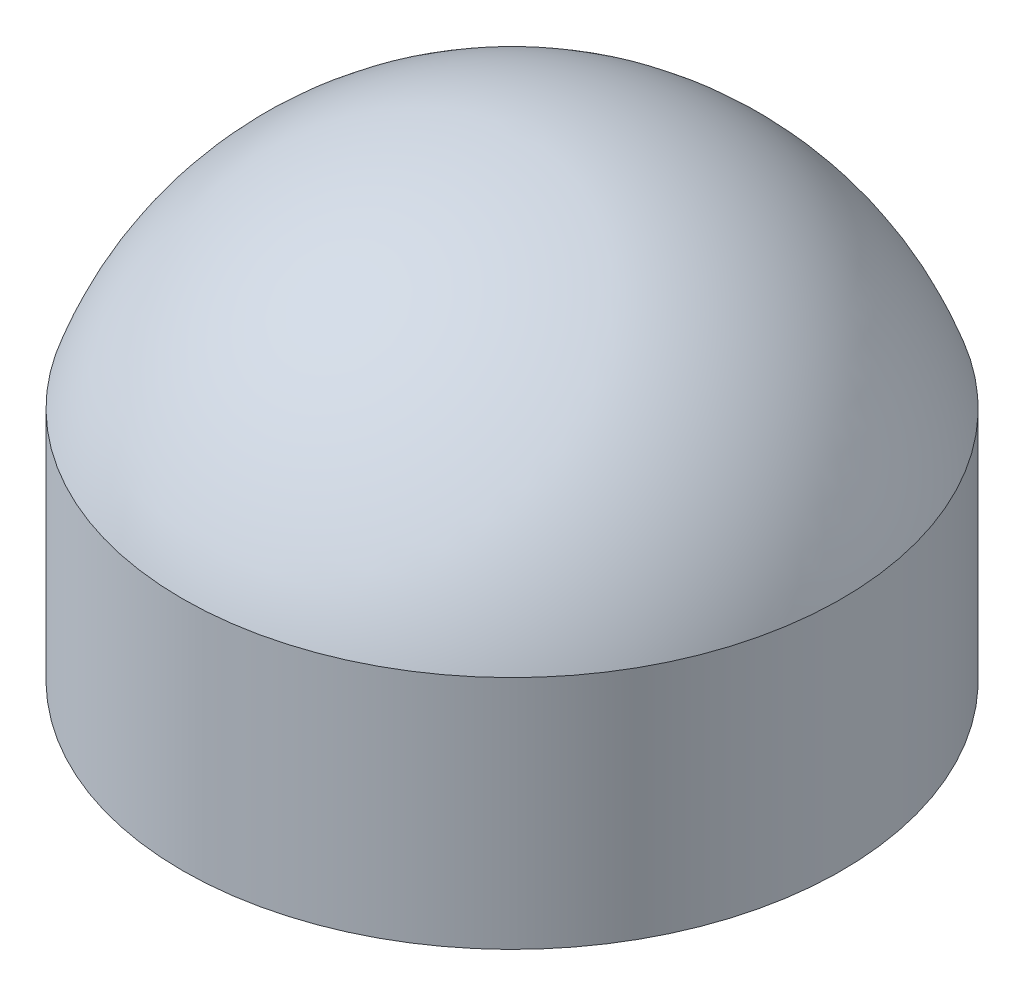
from build123d import *

# Parameters (mm, degrees)
SKETCH1_R           = 70
BOSS_EXTRUDE1_DEPTH = 50
DOME1_FACE_RADIUS   = 70
DOME1_HEIGHT        = 50


with BuildPart() as part:
    # Sketch1 → Boss-Extrude1 (new body)
    with BuildSketch(Plane(origin=(0, 0, 0), x_dir=(1, 0, 0), z_dir=(0, 1, 0))):
        with Locations(Location((0, 0, 0), (0, 0, 270))):
            Circle(SKETCH1_R)
    extrude(amount=BOSS_EXTRUDE1_DEPTH)

    # Dome1: a dome of height H over a round flat face of radius A is a cap of a sphere of radius (A * A + H * H) / (2 * H)
    dome1_r = (DOME1_FACE_RADIUS * DOME1_FACE_RADIUS + DOME1_HEIGHT * DOME1_HEIGHT) / (2 * DOME1_HEIGHT)
    dome1_base = Plane((0, 50, 0), z_dir=(0, 1, 0))
    with Locations(dome1_base.offset(DOME1_HEIGHT - dome1_r)):
        dome1_ball = Sphere(dome1_r, mode=Mode.PRIVATE)
    add(split(dome1_ball, bisect_by=dome1_base, keep=Keep.TOP, mode=Mode.PRIVATE))


solid = part.part
